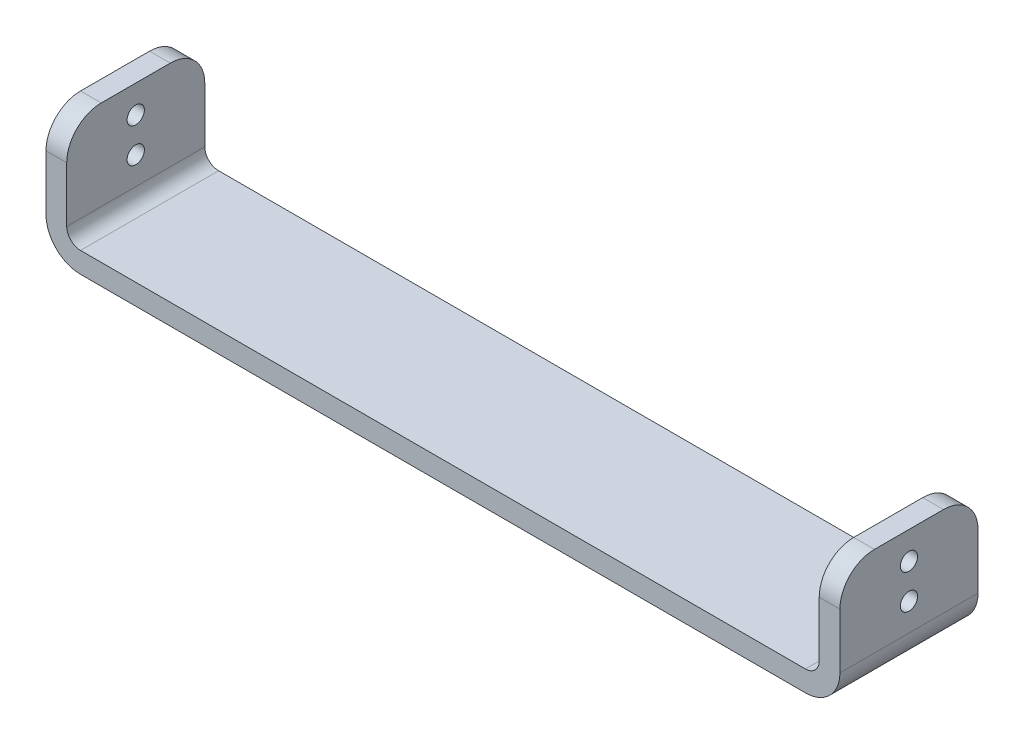
from build123d import *

# Parameters (mm, degrees)
SKETCH1_W           = 115
SKETCH1_H           = 20
BOSS_EXTRUDE1_DEPTH = 3
SKETCH2_W           = 3
SKETCH2_H           = 20
BOSS_EXTRUDE2_DEPTH = 15
FILLET1_R           = 2
FILLET2_R           = 5
M3_TAPPED_HOLE1_D   = 2.5
FILLET3_R           = 5


with BuildPart() as part:
    # Sketch1 → Boss-Extrude1 (new body)
    with BuildSketch(Plane(origin=(0, 0, 0), x_dir=(1, 0, 0), z_dir=(0, 1, 0))):
        Rectangle(SKETCH1_W, SKETCH1_H)
    extrude(amount=BOSS_EXTRUDE1_DEPTH)

    # Sketch2 → Boss-Extrude2 (add)
    with BuildSketch(Plane(origin=(0, 3, 0), x_dir=(1, 0, 0), z_dir=(0, 1, 0))):
        with Locations((-56, 0)):
            Rectangle(SKETCH2_W, SKETCH2_H)
        with Locations((56, 0)):
            Rectangle(SKETCH2_W, SKETCH2_H)
    extrude(amount=BOSS_EXTRUDE2_DEPTH)

    # Fillet1
    fillet1_edges = [part.edges().sort_by_distance(p)[0] for p in [
        (-54.5, 3, 0),
        (54.5, 3, 0),
    ]]
    fillet(fillet1_edges, radius=FILLET1_R)

    # Fillet2
    fillet2_edges = [part.edges().sort_by_distance(p)[0] for p in [
        (-57.5, 0, 0),
        (57.5, 0, 0),
    ]]
    fillet(fillet2_edges, radius=FILLET2_R)

    # M3 Tapped Hole1 (through all)
    with Locations(Plane.ZY.offset(57.5)):
        with Locations((0, 14), (0, 9)):
            Hole(M3_TAPPED_HOLE1_D / 2)

    # Fillet3
    fillet3_edges = [part.edges().sort_by_distance(p)[0] for p in [
        (-56, 18, 10),
        (-56, 18, -10),
        (56, 18, -10),
        (56, 18, 10),
    ]]
    fillet(fillet3_edges, radius=FILLET3_R)


solid = part.part
